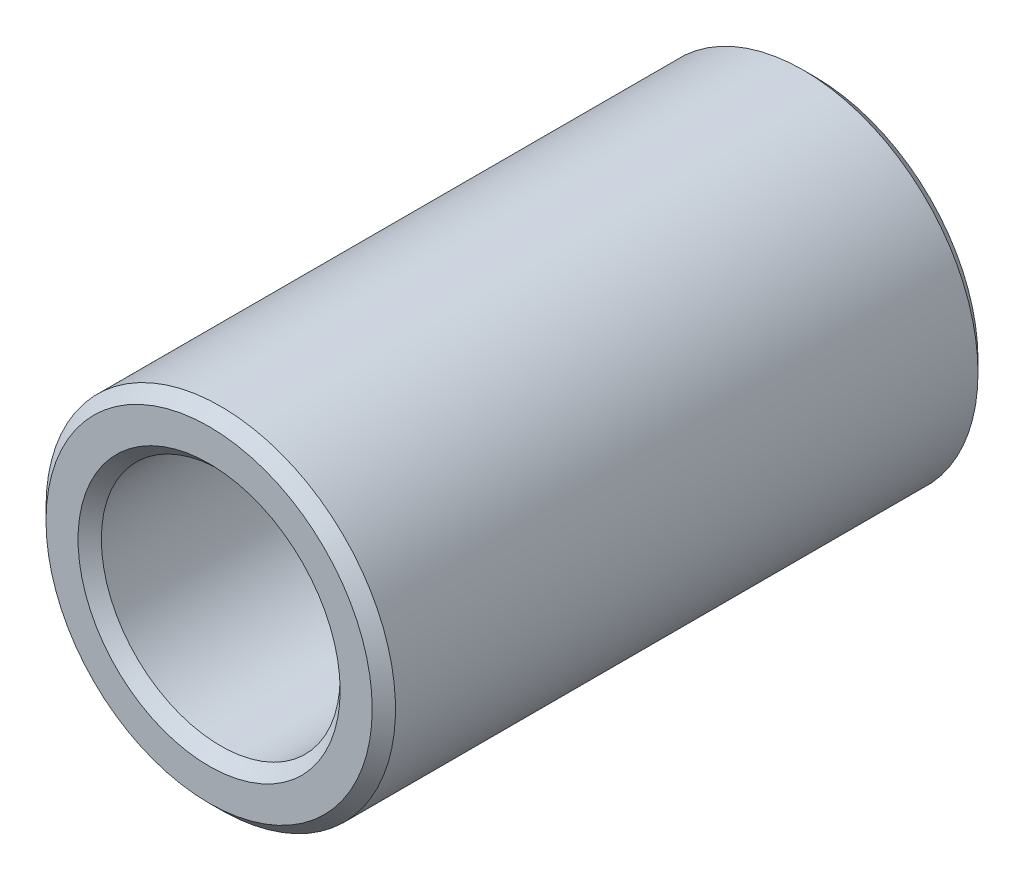
SolidWorks part; units mm, degrees
ref_plane "前视基准面" through (0, 0, 0) normal (0, 0, 1) x (1, 0, 0)
ref_plane "上视基准面" through (0, 0, 0) normal (0, 1, 0) x (1, 0, 0)
ref_plane "右视基准面" through (0, 0, 0) normal (1, 0, 0) x (0, 0, -1)
sketch "草图1" plane through (0, 0, 0) normal (0, 0, 1) x (1, 0, 0)
  circle A0 centre (0, 0) radius 15
  circle A1 centre (0, 0) radius 10.25
  dimension "D1" = 20.5
  dimension "D2" = 30
extrude "凸台-拉伸1" add sketch "草图1" along normal mid plane 52
chamfer "倒角1" distance 1 angle 45 4 edges at (10.25, 0, 26) (10.25, 0, -26) (15, 0, 26) (15, 0, -26)
